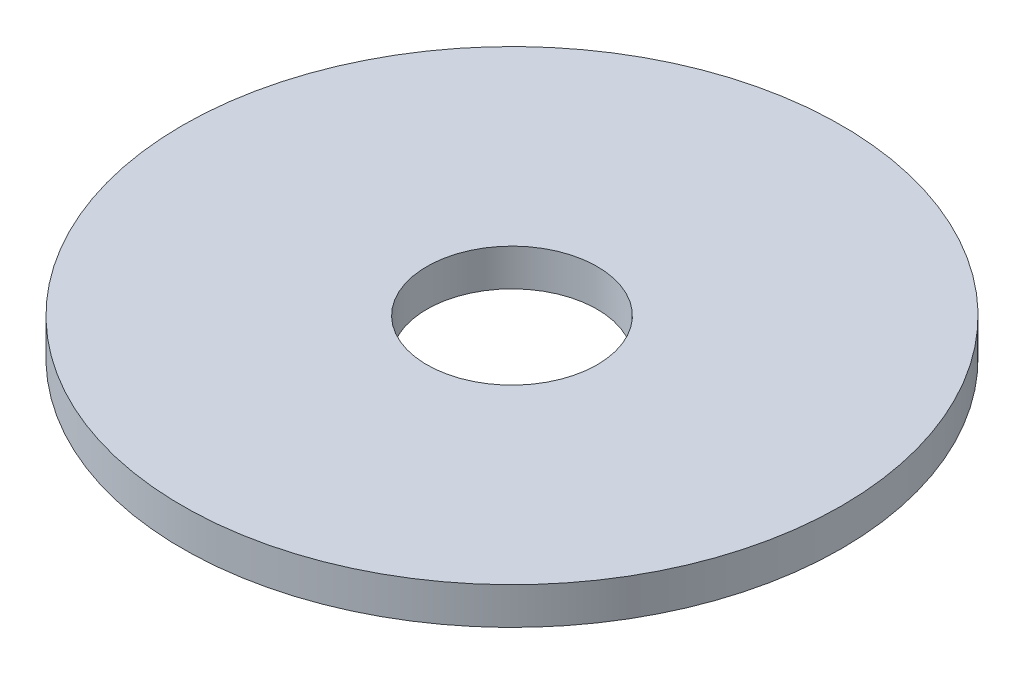
from build123d import *

# Parameters (mm, degrees)
SKETCH1_W = 33
SKETCH1_H = 5


with BuildPart() as part:
    # Sketch1 → Revolve1 (revolve)
    with BuildSketch(Plane.XY):
        with Locations((28, 2.5)):
            Rectangle(SKETCH1_W, SKETCH1_H)
    revolve(axis=Axis((0, -799.868766404, 0), (0, 1, 0)))


solid = part.part
